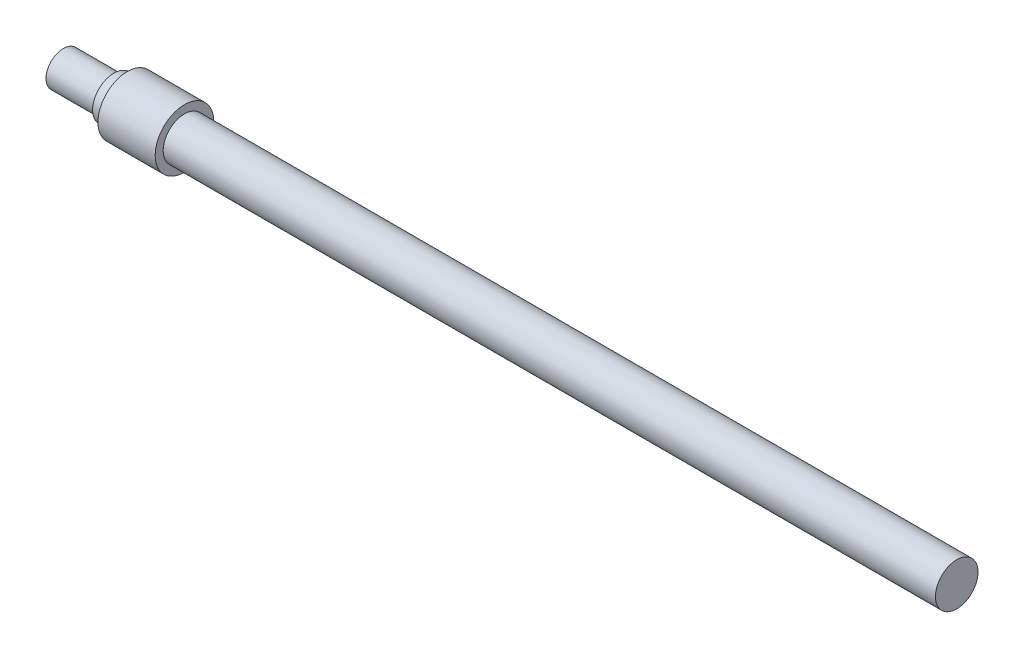
from build123d import *


with BuildPart() as part:
    # 草图1 → 旋转1 (revolve)
    with BuildSketch(Plane.XY, mode=Mode.PRIVATE) as revolve_1_sk:
        Polygon((-108.824631792, 0), (-108.824631792, 13), (-70.824631792, 13), (-70.824631792, 16), (-60.824631792, 16), (-60.824631792, 22), (-17.824631792, 22), (-17.824631792, 16), (562.175368208, 16), (562.175368208, 0), align=None)
    revolve(revolve_1_sk.sketch.rotate(Axis((-119.580443242, 0, 0), (1, 0, 0)), 90), axis=Axis((-119.580443242, 0, 0), (1, 0, 0)))


solid = part.part
